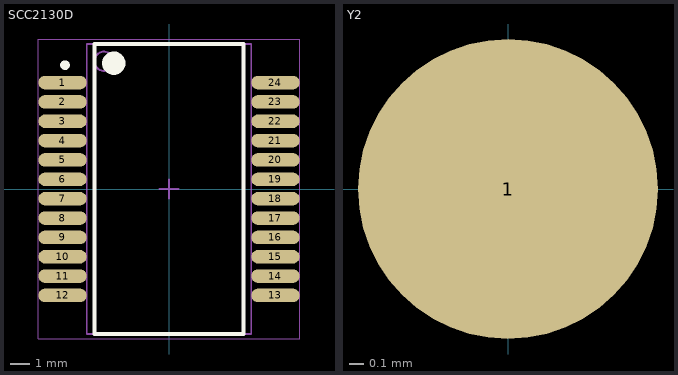
[diagram p0: the footprints below, top view; thin cyan lines are the x and y axes]
# Altium footprint library MISC84456-7.PcbLib: 2 footprints
Each footprint in its own frame and in the unit in brackets; x right, y up, seen from the top. Pads: shape width x height; smd on the part's side, far side on the other; paste and mask are expansions set on the pad; w line width, h text height; cw(c..) or ccw(c..) is an arc to the next point about the centre after c.

## SCC2130D [mm] "SOP, 24-Leads, Body 15.00x8.50mm, Pitch 1.00mm, IPC Medium Density"
height 4.2
pads (24):
  oval 2.5x0.7 smd: 1(-5.5,5.5) 2(-5.5,4.5) 3(-5.5,3.5) 4(-5.5,2.5) 5(-5.5,1.5) 6(-5.5,0.5) 7(-5.5,-0.5) 8(-5.5,-1.5) 9(-5.5,-2.5) 10(-5.5,-3.5) 11(-5.5,-4.5) 12(-5.5,-5.5) 13(5.5,-5.5) 14(5.5,-4.5) 15(5.5,-3.5) 16(5.5,-2.5) 17(5.5,-1.5) 18(5.5,-0.5) 19(5.5,0.5) 20(5.5,1.5) 21(5.5,2.5) 22(5.5,3.5) 23(5.5,4.5) 24(5.5,5.5)
Top Overlay:
  circle w0.25: c-5.375,6.4 r0.125
  circle w0.6: c-2.85,6.5 r0.3
  lines w0.2: -3.85,-7.5 -3.85,7.5 3.85,7.5 3.85,-7.5 -3.85,-7.5
Mechanical 13:
  circle w0.1: c-3.35,6.6 r0.5
  lines w0.1: -4.25,-7.5 -4.25,7.5 4.25,7.5 4.25,-7.5 -4.25,-7.5
Mechanical 15:
  lines w0.05: -6.75,-7.75 -6.75,7.75 6.75,7.75 6.75,-7.75 -6.75,-7.75
  lines w0.1: -0.5,0 0.5,0 ; 0,-0.5 0,0.5
3D body: height 4.2, standoff 0.25, extent -4.25,-7.5 4.25,7.5

## Y2 [mil]
pads (1):
  round 80 smd: 1(0,0)